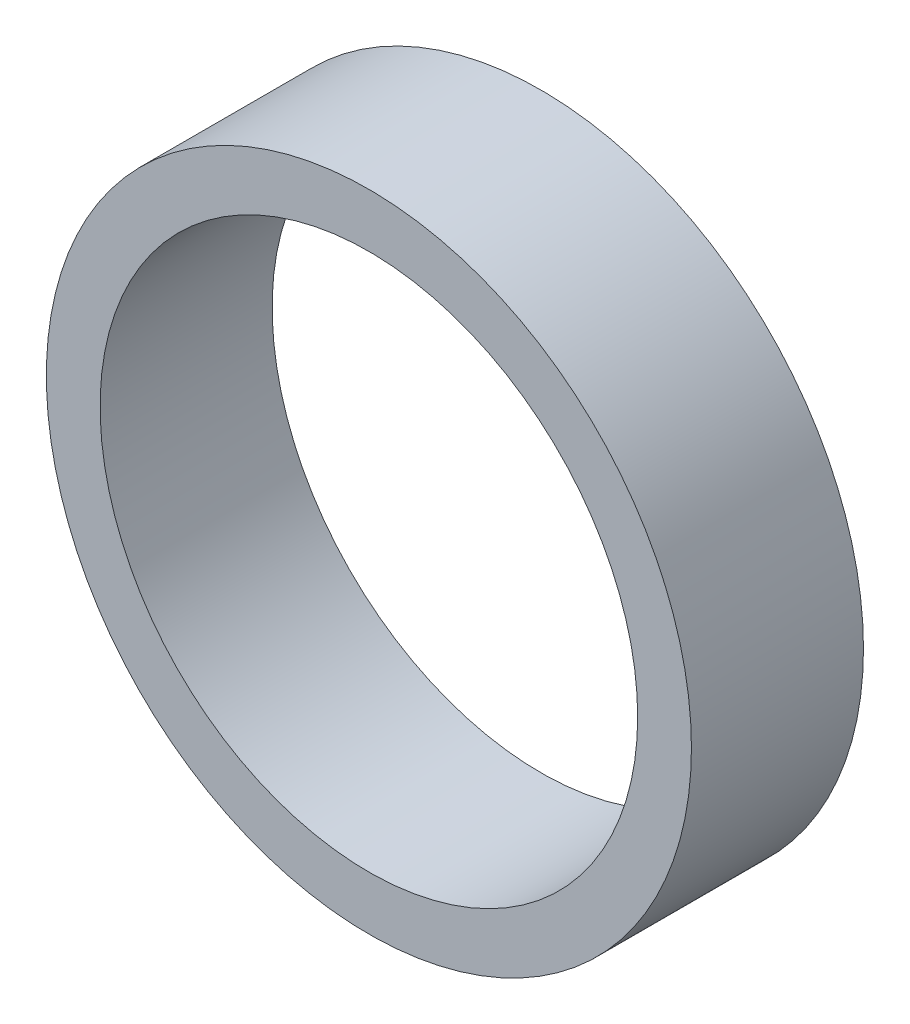
from build123d import *

# Parameters (mm, degrees)
SKETCH_1_R      = 15
SKETCH_1_R_2    = 12.5
EXTRUDE_1_DEPTH = 8


with BuildPart() as part:
    # 草图1 → 凸台-拉伸1 (new body)
    with BuildSketch(Plane.XY):
        Circle(SKETCH_1_R)
        Circle(SKETCH_1_R_2, mode=Mode.SUBTRACT)
    extrude(amount=EXTRUDE_1_DEPTH)


solid = part.part
